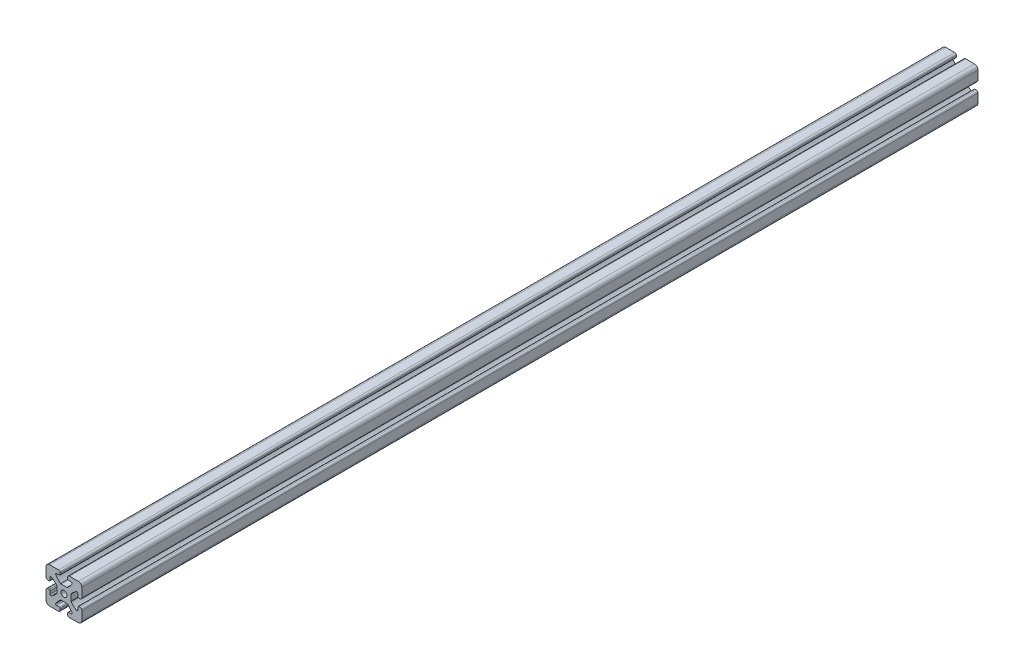
from build123d import *

# Parameters (mm, degrees)
SKETCH1_R           = 3.4
BOSS_EXTRUDE1_DEPTH = 1000


with BuildPart() as part:
    # Sketch1 → Boss-Extrude1 (new body)
    with BuildSketch(Plane.XY):
        with BuildLine():
            Line((-72.552625451, -20.1458069), (-75.708839475, -20.1458069))
            ThreePointArc((-75.708839475, -20.1458069), (-76.585125865, -19.62759748), (-76.55321253, -18.610051226))
            ThreePointArc((-76.55321253, -18.610051226), (-74.186362214, -15.403020453), (-71.332517782, -12.620467892))
            ThreePointArc((-71.332517782, -12.620467892), (-71.036129936, -12.453644757), (-70.700972516, -12.3958069))
            Line((-70.700972516, -12.3958069), (-67.452625451, -12.3958069))
            Line((-67.452625451, -12.3958069), (-64.204278386, -12.3958069))
            ThreePointArc((-64.204278386, -12.3958069), (-63.869120967, -12.453644757), (-63.572733121, -12.620467892))
            ThreePointArc((-63.572733121, -12.620467892), (-60.718888688, -15.403020453), (-58.352038372, -18.610051226))
            ThreePointArc((-58.352038372, -18.610051226), (-58.320125037, -19.62759748), (-59.196411427, -20.1458069))
            Line((-59.196411427, -20.1458069), (-62.352625451, -20.1458069))
            ThreePointArc((-62.352625451, -20.1458069), (-63.059732232, -20.438700119), (-63.352625451, -21.1458069))
            Line((-63.352625451, -21.1458069), (-63.352625451, -22.6458069))
            ThreePointArc((-63.352625451, -22.6458069), (-62.766839013, -24.060020463), (-61.352625451, -24.6458069))
            Line((-61.352625451, -24.6458069), (-51.452625451, -24.6458069))
            ThreePointArc((-51.452625451, -24.6458069), (-48.624198326, -23.474234025), (-47.452625451, -20.6458069))
            Line((-47.452625451, -20.6458069), (-47.452625451, -10.7458069))
            ThreePointArc((-47.452625451, -10.7458069), (-48.038411889, -9.331593338), (-49.452625451, -8.7458069))
            Line((-49.452625451, -8.7458069), (-50.952625451, -8.7458069))
            ThreePointArc((-50.952625451, -8.7458069), (-51.659732232, -9.038700119), (-51.952625451, -9.7458069))
            Line((-51.952625451, -9.7458069), (-51.952625451, -12.902020924))
            ThreePointArc((-51.952625451, -12.902020924), (-52.470834871, -13.778307314), (-53.488381126, -13.74639398))
            ThreePointArc((-53.488381126, -13.74639398), (-56.695411898, -11.379543663), (-59.477964459, -8.525699231))
            ThreePointArc((-59.477964459, -8.525699231), (-59.644787594, -8.229311385), (-59.702625451, -7.894153965))
            Line((-59.702625451, -7.894153965), (-59.702625451, -4.6458069))
            Line((-59.702625451, -4.6458069), (-59.702625451, -1.397459836))
            ThreePointArc((-59.702625451, -1.397459836), (-59.644787594, -1.062302416), (-59.477964459, -0.76591457))
            ThreePointArc((-59.477964459, -0.76591457), (-56.695411898, 2.087929862), (-53.488381126, 4.454780179))
            ThreePointArc((-53.488381126, 4.454780179), (-52.470834871, 4.486693513), (-51.952625451, 3.610407123))
            Line((-51.952625451, 3.610407123), (-51.952625451, 0.4541931))
            ThreePointArc((-51.952625451, 0.4541931), (-51.659732232, -0.252913682), (-50.952625451, -0.5458069))
            Line((-50.952625451, -0.5458069), (-49.452625451, -0.5458069))
            ThreePointArc((-49.452625451, -0.5458069), (-48.038411889, 0.039979537), (-47.452625451, 1.4541931))
            Line((-47.452625451, 1.4541931), (-47.452625451, 11.3541931))
            ThreePointArc((-47.452625451, 11.3541931), (-48.624198326, 14.182620224), (-51.452625451, 15.3541931))
            Line((-51.452625451, 15.3541931), (-61.352625451, 15.3541931))
            ThreePointArc((-61.352625451, 15.3541931), (-62.766839013, 14.768406662), (-63.352625451, 13.3541931))
            Line((-63.352625451, 13.3541931), (-63.352625451, 11.8541931))
            ThreePointArc((-63.352625451, 11.8541931), (-63.059732232, 11.147086318), (-62.352625451, 10.8541931))
            Line((-62.352625451, 10.8541931), (-59.196411427, 10.8541931))
            ThreePointArc((-59.196411427, 10.8541931), (-58.320125037, 10.335983679), (-58.352038372, 9.318437425))
            ThreePointArc((-58.352038372, 9.318437425), (-60.718888688, 6.111406652), (-63.572733121, 3.328854091))
            ThreePointArc((-63.572733121, 3.328854091), (-63.869120967, 3.162030956), (-64.204278386, 3.1041931))
            Line((-64.204278386, 3.1041931), (-67.452625451, 3.1041931))
            Line((-67.452625451, 3.1041931), (-70.700972516, 3.1041931))
            ThreePointArc((-70.700972516, 3.1041931), (-71.036129936, 3.162030956), (-71.332517782, 3.328854091))
            ThreePointArc((-71.332517782, 3.328854091), (-74.186362214, 6.111406652), (-76.55321253, 9.318437425))
            ThreePointArc((-76.55321253, 9.318437425), (-76.585125865, 10.335983679), (-75.708839475, 10.8541931))
            Line((-75.708839475, 10.8541931), (-72.552625451, 10.8541931))
            ThreePointArc((-72.552625451, 10.8541931), (-71.84551867, 11.147086318), (-71.552625451, 11.8541931))
            Line((-71.552625451, 11.8541931), (-71.552625451, 13.3541931))
            ThreePointArc((-71.552625451, 13.3541931), (-72.138411889, 14.768406662), (-73.552625451, 15.3541931))
            Line((-73.552625451, 15.3541931), (-83.452625451, 15.3541931))
            ThreePointArc((-83.452625451, 15.3541931), (-86.281052576, 14.182620224), (-87.452625451, 11.3541931))
            Line((-87.452625451, 11.3541931), (-87.452625451, 1.4541931))
            ThreePointArc((-87.452625451, 1.4541931), (-86.866839013, 0.039979537), (-85.452625451, -0.5458069))
            Line((-85.452625451, -0.5458069), (-83.952625451, -0.5458069))
            ThreePointArc((-83.952625451, -0.5458069), (-83.24551867, -0.252913682), (-82.952625451, 0.4541931))
            Line((-82.952625451, 0.4541931), (-82.952625451, 3.610407123))
            ThreePointArc((-82.952625451, 3.610407123), (-82.434416031, 4.486693513), (-81.416869776, 4.454780179))
            ThreePointArc((-81.416869776, 4.454780179), (-78.209839004, 2.087929862), (-75.427286443, -0.76591457))
            ThreePointArc((-75.427286443, -0.76591457), (-75.260463308, -1.062302416), (-75.202625451, -1.397459836))
            Line((-75.202625451, -1.397459836), (-75.202625451, -4.6458069))
            Line((-75.202625451, -4.6458069), (-75.202625451, -7.894153965))
            ThreePointArc((-75.202625451, -7.894153965), (-75.260463308, -8.229311385), (-75.427286443, -8.525699231))
            ThreePointArc((-75.427286443, -8.525699231), (-78.209839004, -11.379543663), (-81.416869776, -13.74639398))
            ThreePointArc((-81.416869776, -13.74639398), (-82.434416031, -13.778307314), (-82.952625451, -12.902020924))
            Line((-82.952625451, -12.902020924), (-82.952625451, -9.7458069))
            ThreePointArc((-82.952625451, -9.7458069), (-83.24551867, -9.038700119), (-83.952625451, -8.7458069))
            Line((-83.952625451, -8.7458069), (-85.452625451, -8.7458069))
            ThreePointArc((-85.452625451, -8.7458069), (-86.866839013, -9.331593338), (-87.452625451, -10.7458069))
            Line((-87.452625451, -10.7458069), (-87.452625451, -20.6458069))
            ThreePointArc((-87.452625451, -20.6458069), (-86.281052576, -23.474234025), (-83.452625451, -24.6458069))
            Line((-83.452625451, -24.6458069), (-73.552625451, -24.6458069))
            ThreePointArc((-73.552625451, -24.6458069), (-72.138411889, -24.060020463), (-71.552625451, -22.6458069))
            Line((-71.552625451, -22.6458069), (-71.552625451, -21.1458069))
            ThreePointArc((-71.552625451, -21.1458069), (-71.84551867, -20.438700119), (-72.552625451, -20.1458069))
        make_face()
        with Locations((-67.452625451, -4.6458069)):
            Circle(SKETCH1_R, mode=Mode.SUBTRACT)
    extrude(amount=BOSS_EXTRUDE1_DEPTH)


solid = part.part
